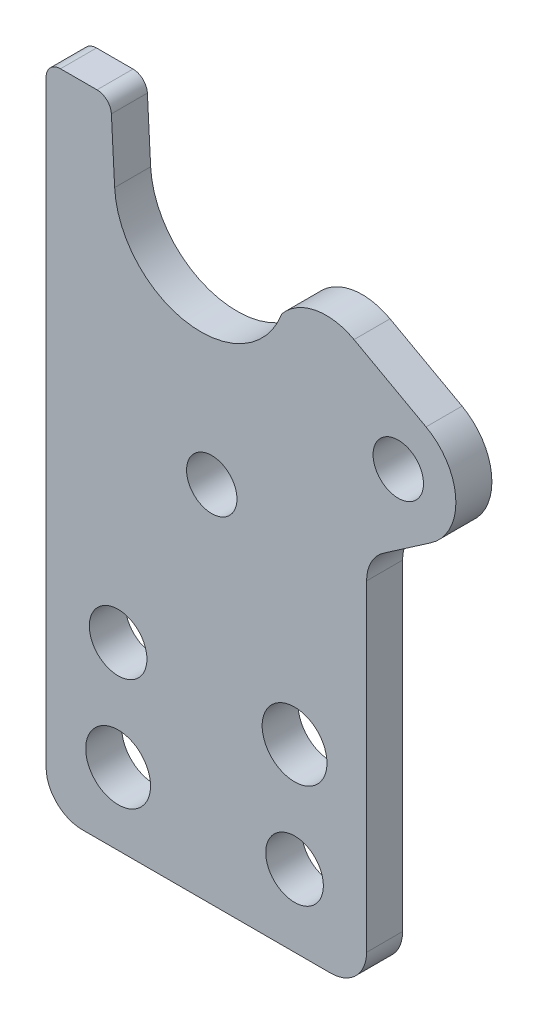
from build123d import *

# Parameters (mm, degrees)
SKETCH1_R           = 3.5
SKETCH1_R_2         = 4.5
SKETCH1_R_3         = 4
BOSS_EXTRUDE1_DEPTH = 5
FILLET1_R           = 2
FILLET2_R           = 5


with BuildPart() as part:
    # Sketch1 → Boss-Extrude1 (new body)
    with BuildSketch(Plane.XY):
        with BuildLine():
            Line((8.964694833, 90), (9.516445583, 79.471968525))
            ThreePointArc((9.516445583, 79.471968525), (19.681156059, 68.23864229), (32.744762205, 75.910092728))
            ThreePointArc((32.744762205, 75.910092728), (37.408516237, 78.659737666), (42.755349998, 77.809727269))
            Line((42.755349998, 77.809727269), (52.755349998, 72.309727269))
            ThreePointArc((52.755349998, 72.309727269), (56.88996042, 65.700665064), (53.437266153, 58.711129395))
            Line((53.437266153, 58.711129395), (46.88062952, 54.196060385))
            ThreePointArc((46.88062952, 54.196060385), (45.131399706, 52.224869926), (44.5, 49.666211844))
            Line((44.5, 49.666211844), (44.5, 0))
            Line((44.5, 0), (0, 0))
            Line((0, 0), (0, 90))
            Line((0, 90), (8.964694833, 90))
        make_face()
        with Locations((48.9, 65.3)):
            Circle(SKETCH1_R, mode=Mode.SUBTRACT)
        with Locations((10, 10)):
            Circle(SKETCH1_R_2, mode=Mode.SUBTRACT)
        with Locations((10, 25)):
            Circle(SKETCH1_R_3, mode=Mode.SUBTRACT)
        with Locations((34.5, 10)):
            Circle(SKETCH1_R_3, mode=Mode.SUBTRACT)
        with Locations((34.5, 25)):
            Circle(SKETCH1_R_2, mode=Mode.SUBTRACT)
        with Locations((23, 50.5)):
            Circle(SKETCH1_R, mode=Mode.SUBTRACT)
    extrude(amount=BOSS_EXTRUDE1_DEPTH)

    # Fillet1
    fillet1_edges = [part.edges().sort_by_distance(p)[0] for p in [
        (0, 90, 2.5),
        (8.964694833, 90, 2.5),
    ]]
    fillet(fillet1_edges, radius=FILLET1_R)

    # Fillet2
    fillet2_edges = [part.edges().sort_by_distance(p)[0] for p in [
        (44.5, 0, 2.5),
        (0, 0, 2.5),
    ]]
    fillet(fillet2_edges, radius=FILLET2_R)


solid = part.part
